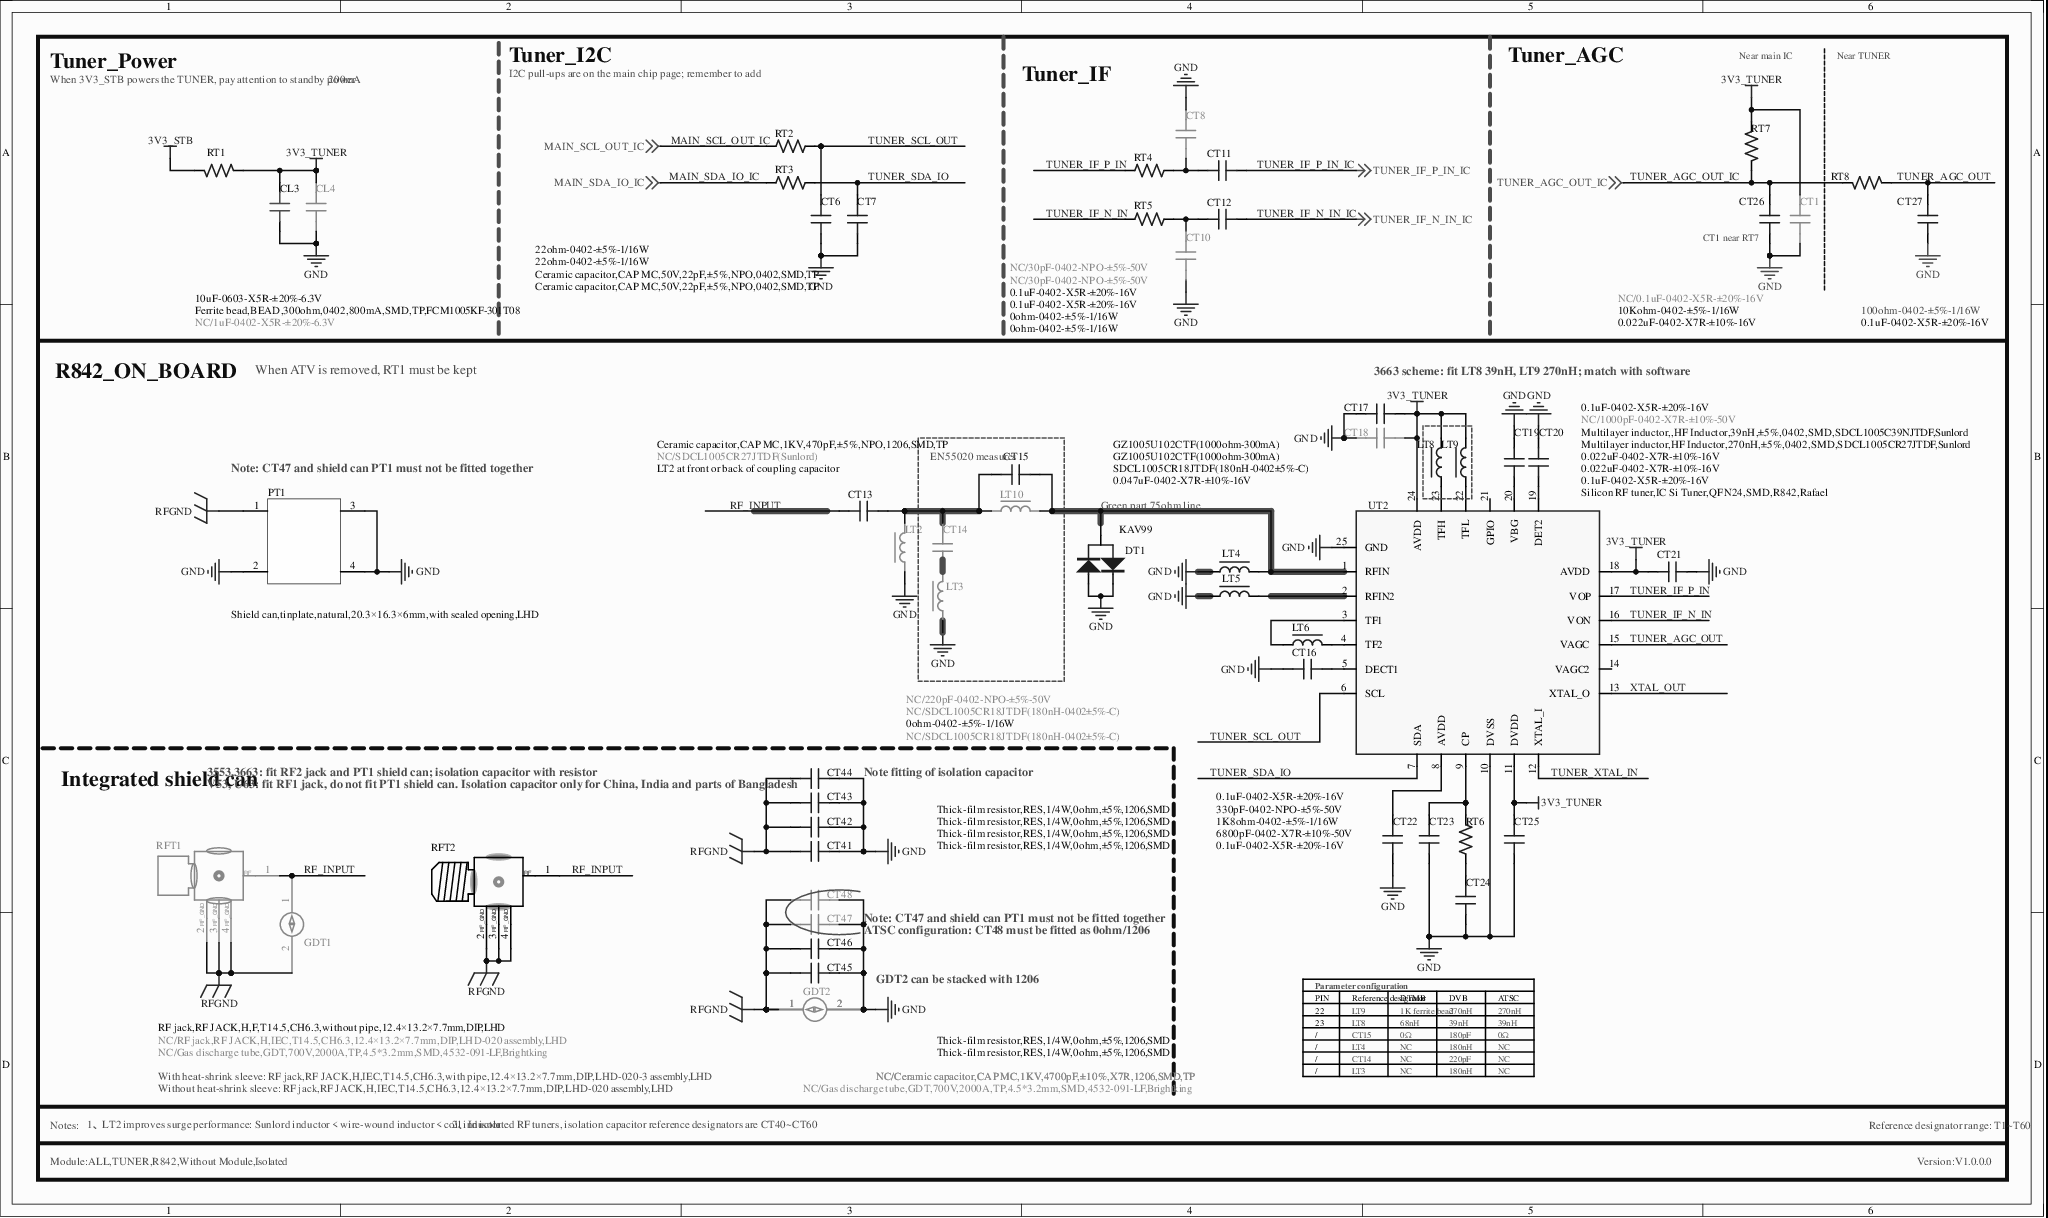
[diagram p0: MISC86372-16.SchDoc]
# Altium project MISC86372-32.PrjPCB (part 6 of 8)

## Sheet MISC86372-16.SchDoc
size 426 x 254 mm

### Parts
CL3  10uF-0603-X5R-±20%-6.3V  [C0603]
CL4  NC/1uF-0402-X5R-±20%-6.3V  [C0402]
CT1  NC/0.1uF-0402-X5R-±20%-16V  [C0402]
CT6  Ceramic capacitor,CAP MC,50V,22pF,±5%,NPO,0402,SMD,TP  [C0402]
CT7  Ceramic capacitor,CAP MC,50V,22pF,±5%,NPO,0402,SMD,TP  [C0402]
CT8  NC/30pF-0402-NPO-±5%-50V  [C0402]
CT10  NC/30pF-0402-NPO-±5%-50V  [C0402]
CT11  0.1uF-0402-X5R-±20%-16V  [C0402]
CT12  0.1uF-0402-X5R-±20%-16V  [C0402]
CT13  Ceramic capacitor,CAP MC,1KV,470pF,±5%,NPO,1206,SMD,TP  [C1206]
CT14  NC/220pF-0402-NPO-±5%-50V  [C0402]
CT15  0ohm-0402-±5%-1/16W  [C0402]
CT16  0.047uF-0402-X7R-±10%-16V  [C0402]
CT17  0.1uF-0402-X5R-±20%-16V  [C0402]
CT18  NC/1000pF-0402-X7R-±10%-50V  [C0402]
CT19  0.022uF-0402-X7R-±10%-16V  [C0402]
CT20  0.022uF-0402-X7R-±10%-16V  [C0402]
CT21  0.1uF-0402-X5R-±20%-16V  [C0402]
CT22  0.1uF-0402-X5R-±20%-16V  [C0402]
CT23  330pF-0402-NPO-±5%-50V  [C0402]
CT24  6800pF-0402-X7R-±10%-50V  [C0402]
CT25  0.1uF-0402-X5R-±20%-16V  [C0402]
CT26  0.022uF-0402-X7R-±10%-16V  [C0402]
CT27  0.1uF-0402-X5R-±20%-16V  [C0402]
CT41  Thick-film resistor,RES,1/4W,0ohm,±5%,1206,SMD  [C1206]
CT42  Thick-film resistor,RES,1/4W,0ohm,±5%,1206,SMD  [C1206]
CT43  Thick-film resistor,RES,1/4W,0ohm,±5%,1206,SMD  [C1206]
CT44  Thick-film resistor,RES,1/4W,0ohm,±5%,1206,SMD  [C1206]
CT45  Thick-film resistor,RES,1/4W,0ohm,±5%,1206,SMD  [C1206]
CT46  Thick-film resistor,RES,1/4W,0ohm,±5%,1206,SMD  [C1206]
CT47  NC/Ceramic capacitor,CAP MC,1KV,4700pF,±10%,X7R,1206,SMD,TP  [C1206]
CT48  NC/Ceramic capacitor,CAP MC,1KV,4700pF,±10%,X7R,1206,SMD,TP  [C1206]
DT1  KAV99  [SO-23]
GDT1  NC/Gas discharge tube,GDT,700V,2000A,TP,4.5*3.2mm,SMD,4532-091-LF,Brightking  [SMD4532-1]
GDT2  NC/Gas discharge tube,GDT,700V,2000A,TP,4.5*3.2mm,SMD,4532-091-LF,Brightking  [SMD4532-1-C1206]
LT2  NC/SDCL1005CR27JTDF(Sunlord)  [L0402]
LT3  NC/SDCL1005CR18JTDF(180nH-0402±5%-C)  [L0402]
LT4  GZ1005U102CTF(1000ohm-300mA)  [L0402]
LT5  GZ1005U102CTF(1000ohm-300mA)  [L0402]
LT6  SDCL1005CR18JTDF(180nH-0402±5%-C)  [L0402]
LT8  Multilayer inductor,,HF Inductor,39nH,±5%,0402,SMD,SDCL1005C39NJTDF,Sunlord  [L0402]
LT9  Multilayer inductor,HF Inductor,270nH,±5%,0402,SMD,SDCL1005CR27JTDF,Sunlord  [L0402]
LT10  NC/SDCL1005CR18JTDF(180nH-0402±5%-C)  [L0402]
PT1  Shield can,tinplate,natural,20.3×16.3×6mm,with sealed opening,LHD  [SHIELD(16*20*6)]
RFT1  NC/RF jack,RF JACK,H,IEC,T14.5,CH6.3,12.4×13.2×7.7mm,DIP,LHD-020 assembly,LHD  [ANT-IEC14.5-H-4]
RFT2  RF jack,RF JACK,H,F,T14.5,CH6.3,without pipe,12.4×13.2×7.7mm,DIP,LHD  [T-13.2×12.4×7.7-F14.5]
RT1  Ferrite bead,BEAD,300ohm,0402,800mA,SMD,TP,FCM1005KF-301T08  [R0402]
RT2  22ohm-0402-±5%-1/16W  [R0402]
RT3  22ohm-0402-±5%-1/16W  [R0402]
RT4  0ohm-0402-±5%-1/16W  [R0402]
RT5  0ohm-0402-±5%-1/16W  [R0402]
RT6  1K8ohm-0402-±5%-1/16W  [R0402]
RT7  10Kohm-0402-±5%-1/16W  [R0402]
RT8  100ohm-0402-±5%-1/16W  [R0402]
UT2  Silicon RF tuner,IC Si Tuner,QFN24,SMD,R842,Rafael  [QFN24/0.5-3]

### Blocks framed on the sheet
EN55020 measures: CT14 CT15 LT3 LT10

### Nets
3V3_STB: RT1.2
3V3_TUNER: CL3.2 CL4.2 CT1.1 CT17.2 CT18.1 CT21.2 CT25.1 LT8.1 LT9.2 RT1.1 RT7.1 UT2.11(DVDD) UT2.18(AVDD) UT2.24(AVDD)
GND: CL3.1 CL4.1 CT1.2 CT6.1 CT7.1 CT8.1 CT10.2 CT16.2 CT17.1 CT18.2 CT19.1 CT20.2 CT21.1 CT22.2 CT23.1 CT24.1 CT25.2 CT26.1 CT27.1 CT41.1 CT42.1 CT43.1 CT44.1 CT45.1 CT46.1 CT47.1 CT48.1 DT1.1 DT1.3 GDT2.2 LT2.2 LT3.2 LT4.2 LT5.2 PT1.2 PT1.3 PT1.4 UT2.10(DVSS) UT2.25(GND)
RFGND: CT41.2 CT42.2 CT43.2 CT44.2 CT45.2 CT46.2 CT47.2 CT48.2 GDT1.2 GDT2.1 PT1.1 RFT1.2 RFT1.3 RFT1.4 RFT2.2 RFT2.3 RFT2.4
MAIN_SCL_OUT_IC: RT2.1 ; off-sheet MAIN_SCL_OUT_IC
MAIN_SDA_IO_IC: RT3.1 ; off-sheet MAIN_SDA_IO_IC
RF_INPUT: CT13.1 GDT1.1 RFT1.1 RFT2.1
TUNER_AGC_OUT: CT27.2 RT8.1 UT2.15(VAGC)
TUNER_AGC_OUT_IC: CT26.2 RT7.2 RT8.2 ; off-sheet TUNER_AGC_OUT_IC
TUNER_IF_N_IN: RT5.1 UT2.16(VON)
TUNER_IF_N_IN_IC: CT12.1 ; off-sheet TUNER_IF_N_IN_IC
TUNER_IF_P_IN: RT4.1 UT2.17(VOP)
TUNER_IF_P_IN_IC: CT11.1 ; off-sheet TUNER_IF_P_IN_IC
TUNER_SCL_OUT: CT6.2 RT2.2 UT2.6(SCL)
TUNER_SDA_IO: CT7.2 RT3.2 UT2.7(SDA)
TUNER_XTAL_IN: UT2.12(XTAL_I)
XTAL_OUT: UT2.13(XTAL_O)
NetCT8_2: CT8.2 CT11.2 RT4.2
NetCT10_1: CT10.1 CT12.2 RT5.2
NetCT13_2: CT13.2 CT14.1 CT15.1 LT2.1 LT10.2
NetCT14_2: CT14.2 LT3.1
NetCT15_2: CT15.2 DT1.2 LT4.1 LT10.1 UT2.1(RFIN)
NetCT16_1: CT16.1 UT2.5(DECT1)
NetCT19_2: CT19.2 UT2.20(VBG)
NetCT20_1: CT20.1 UT2.19(DET2)
NetCT22_1: CT22.1 UT2.8(AVDD)
NetCT23_2: CT23.2 RT6.2 UT2.9(CP)
NetCT24_2: CT24.2 RT6.1
NetLT5_1: LT5.1 UT2.2(RFIN2)
NetLT6_1: LT6.1 UT2.4(TF2)
NetLT6_2: LT6.2 UT2.3(TF1)
NetLT8_2: LT8.2 UT2.23(TFH)
NetLT9_1: LT9.1 UT2.22(TFL)

Not connected (* = marked no-connect by the designer): UT2 14(VAGC2)* 21(GPIO)*

### Notes on the sheet
- Tuner_Power
- When 3V3_STB powers the TUNER, pay attention to standby power
- 200mA
- Tuner_I2C
- I2C pull-ups are on the main chip page; remember to add
- Tuner_IF
- Tuner_AGC
- Near main IC
- Near TUNER
- (near CT26) CT1 near RT7
- R842_ON_BOARD
- When ATV is removed, RT1 must be kept
- (near CT17) 3663 scheme: fit LT8 39nH, LT9 270nH; match with software
- (near PT1) Note: CT47 and shield can PT1 must not be fitted together
- (near CT13) LT2 at front or back of coupling capacitor
- (near DT1) Green part 75ohm line
- Integrated shield can
- 3553,3663: fit RF2 jack and PT1 shield can; isolation capacitor with resistor
- (near CT44) V53, U63: fit RF1 jack, do not fit PT1 shield can. Isolation capacitor only for China, India and parts of Bangladesh
- Note fitting of isolation capacitor
- Note: CT47 and shield can PT1 must not be fitted together
- ATSC configuration: CT48 must be fitted as 0ohm/1206
- GDT2 can be stacked with 1206
- PIN
- Parameter configuration
- Reference designator
- DTMB
- DVB
- ATSC
- 22
- 23
- /
- LT9
- LT8
- CT15
- LT4
- 1K ferrite bead
- 68nH
- 0Ω
- NC
- 270nH
- 39nH
- 180pF
- 180nH
- Without heat-shrink sleeve: RF jack,RF JACK,H,IEC,T14.5,CH6.3,12.4×13.2×7.7mm,DIP,LHD-020 assembly,LHD
- With heat-shrink sleeve: RF jack,RF JACK,H,IEC,T14.5,CH6.3,with pipe,12.4×13.2×7.7mm,DIP,LHD-020-3 assembly,LHD
- CT14
- LT3
- 220pF
- Module:ALL,TUNER,R842,Without Module,Isolated
- Notes:
- 1、 LT2 improves surge performance: Sunlord inductor < wire-wound inductor < coil inductor
- 2、 In isolated RF tuners, isolation capacitor reference designators are CT40~CT60
- Reference designator range: T1~T60
- Version:V1.0.0.0

### Library data of the parts
CL3 = 004.003.0000383-D: Ceramic capacitor,CAP MC,6.3V,10uF,±20%,X5R,0603,SMD,TP-D
CL4 = 004.003.0000382-D: Ceramic capacitor,CAP MC,6.3V,1uF,±20%,X5R,0402,SMD,TP-D
CT1 CT11 CT12 CT17 = 004.003.0000403-D: Ceramic capacitor,CAP MC,16V,0.1uF,±20%,X5R,0402,SMD,TP-D
CT6 CT7 = 004.003.0000530-D: Ceramic capacitor,CAP MC,50V,22pF,±5%,NPO,0402,SMD,TP-D
CT8 CT10 = 004.003.0000556-D: Ceramic capacitor,CAP MC,50V,47pF,±5%,NPO,0402,SMD,TP-D
CT13 = 0.47uF-1206-Y5V-+80%-20%-16V-D
CT14 = 220pF-0402-NPO-±5%-50V-D
CT15 = 180pF-0402-NPO-±5%-50V-D
CT16 = 0.047uF-0402-X7R-±10%-16V-D
CT18 = 1000pF-0402-X7R-±10%-50V-D
CT19 CT21 CT22 CT25 = 0.1uF-0402-X5R-±20%-16V-D
CT20 CT26 = 0.022uF-0402-X7R-±10%-16V-D
CT23 = 330pF-0402-NPO-±5%-50V-D
CT24 = 6800pF-0402-X7R-±10%-50V-D
CT27 = 0.1uF-0402-Y5V-+80%-20%-16V-D
CT41 CT43-CT45 CT47 CT48 = 1000pF-1206-X7R-±20%-2000V-D
CT42 CT46 = 1000pF-1206-X7R±10%-2000V-D
DT1 = 004.005.0000195-D: Switching diode,DIO SW D2,200mA,70V,SOT-23,SMD,BAV99,BLUE ROCKET-D
GDT1 = 004.005.0000675: Gas discharge tube,GDT,700V,2000A,TP,4.5*3.2mm,SMD,4532-091-LF,Brightking-D
GDT2 = 004.005.0000675-C1206: Gas discharge tube,GDT,700V,2000A,TP,4.5*3.2mm,SMD,4532-091-LF,Brightking-D
LT2 = SDCL1005CR27JTDF(顺络)-D
LT3 LT6 LT10 = 004.004.0000087-D: Multilayer inductor,HF Inductor,180nH,±5%,0402,SMD,SDCL1005CR18JTDF,Sunlord-D
LT4 LT5 = GZ1005U102CTF(1000ohm-300mA)-D
LT8 = SDCL1005C68NJTDF(68nH-0402±5%-C)-D
LT9 = 1Kohm-0402-±25%-D
PT1 = 004.040.0000768-DMI: Shield can,tinplate,natural,20.3×16.3×6mm,with sealed opening,LHD-DMI
RFT1 = RF头,RF JACK,H,IEC,T14.5,CH6.3,12.4×13.2×7.7mm,DIP,LHD-020组件,LHD-DLMI: T-IEC-6.3mm-#-#
RFT2 = RF头,RF JACK,H,F,T14.5,CH6.3,without pipe,12.4×13.2×7.7mm,DIP,LHD-DLMI: T-F-6.3mm-#-#
RT1 = 004.002.0000558-D: Thick-film resistor,RES,1/16W,0ohm,±5%,0402,SMD-D
RT2 RT3 = 22ohm-0402-±5%-1/16W-D
RT4 RT5 = 0ohm-0402-±5%-1/16W-D
RT6 = 1K8ohm-0402-±5%-1/16W-D
RT7 RT8 = 10Kohm-0402-±5%-1/16W-D
UT2 = 硅高频头,IC Si Tuner,QFN24,SMD,R842,Rafael-D